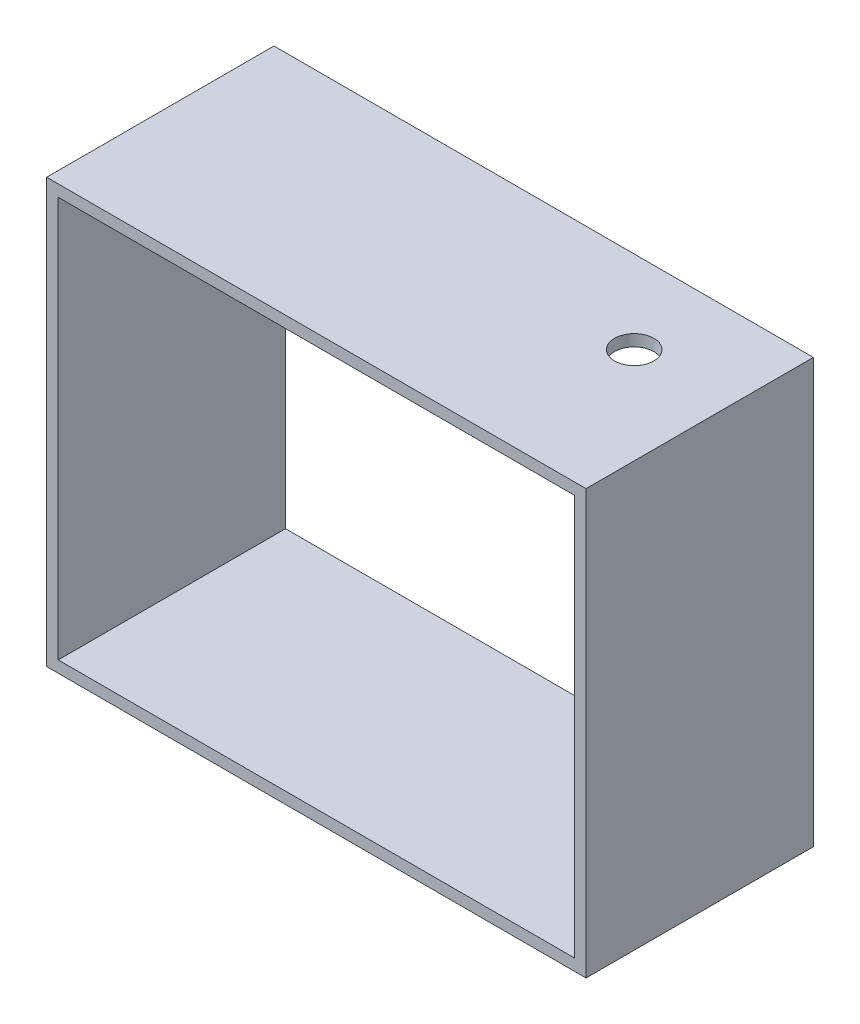
SolidWorks part; units mm, degrees
ref_plane "前视基准面" through (0, 0, 0) normal (0, 0, 1) x (1, 0, 0)
ref_plane "上视基准面" through (0, 0, 0) normal (0, 1, 0) x (1, 0, 0)
ref_plane "右视基准面" through (0, 0, 0) normal (1, 0, 0) x (0, 0, -1)
other "Configuration Table"
sketch "草图1" plane through (0, 0, 0) normal (0, 0, 1) x (1, 0, 0)
  line L0 (-70, -55) -> (70, -55)
  line L1 (70, -55) -> (70, 55)
  line L2 (70, 55) -> (-70, 55)
  line L3 (-70, 55) -> (-70, -55)
  line L4 (-67, -52) -> (67, -52)
  line L5 (67, -52) -> (67, 52)
  line L6 (67, 52) -> (-67, 52)
  line L7 (-67, 52) -> (-67, -52)
  point P0 (0, 0)
  dimension "D1" = 3
  dimension "D2" = 70
  dimension "D3" = 137
  dimension "D4" = 140
  dimension "D5" = 3
  dimension "D6" = 55
  dimension "D7" = 107
  dimension "D8" = 110
extrude "凸台-拉伸1" add sketch "草图1" against normal mid plane 59
sketch "草图2" plane through (0, 0, 0) normal (0, 1, 0) x (1, 0, 0)
  circle A0 centre (45, 8) radius 5.1
  point P0 (0, 0)
  dimension "D1" = 10.2
  dimension "D2" = 45
  dimension "D3" = 8
extrude "切除-拉伸1" cut sketch "草图2" against normal mid plane 140
